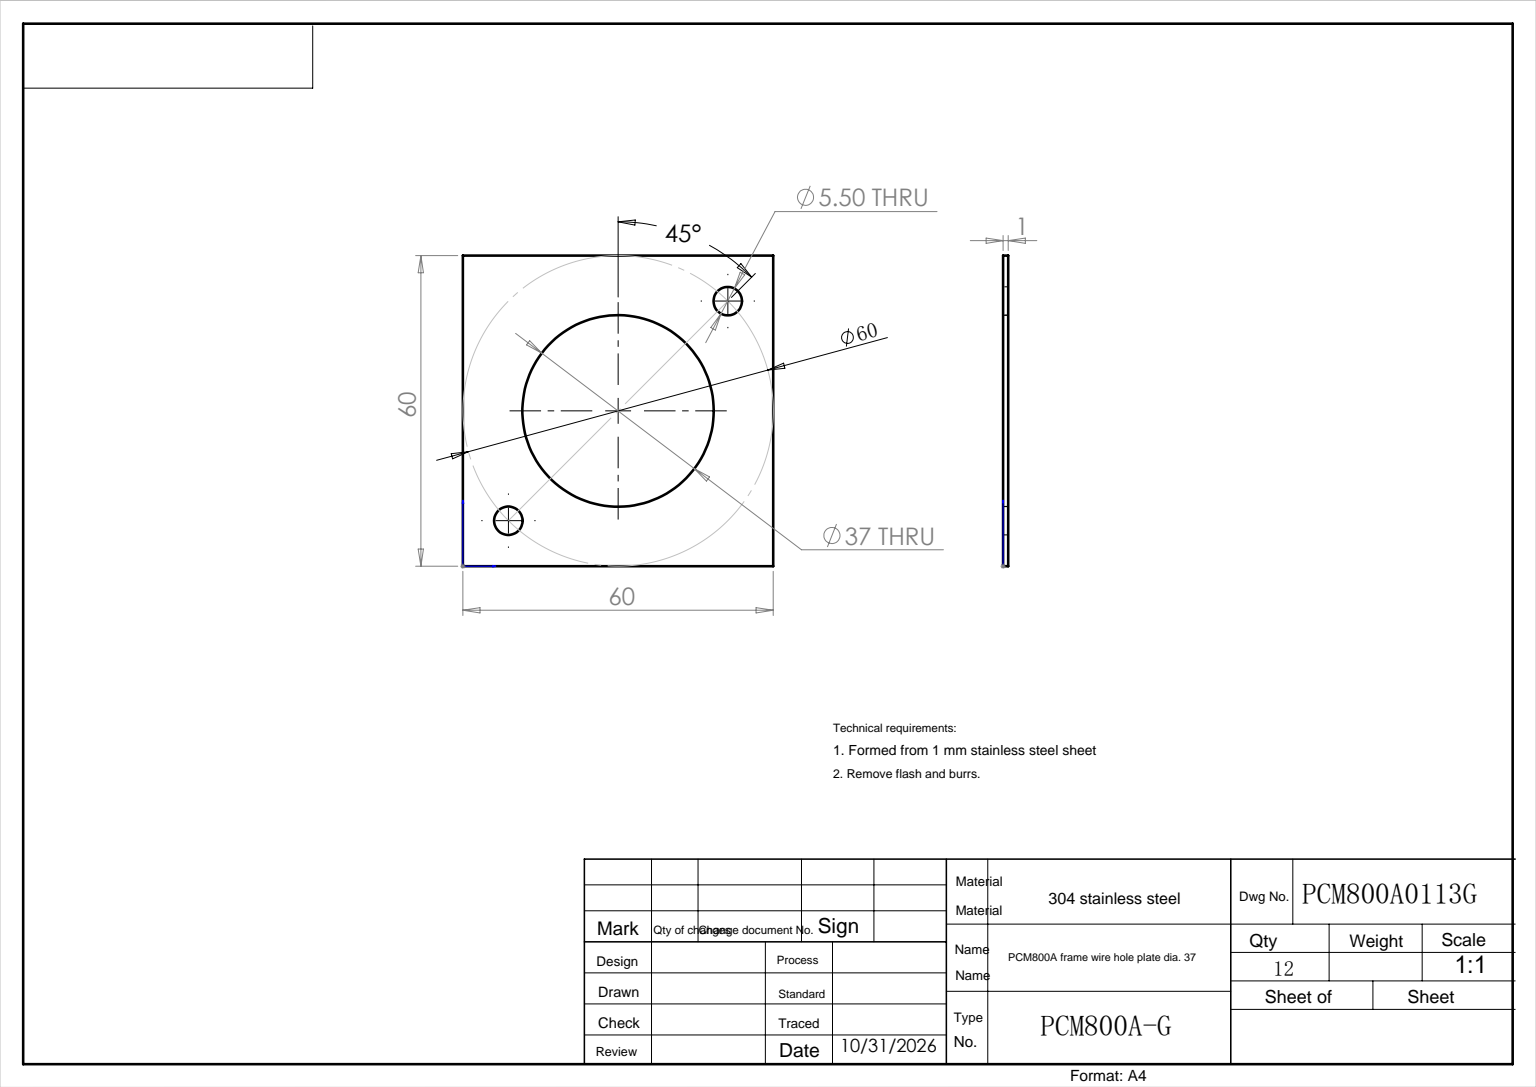
SolidWorks part; units mm, degrees
ref_plane "前视基准面" through (0, 0, 0) normal (0, 0, 1) x (1, 0, 0)
ref_plane "上视基准面" through (0, 0, 0) normal (0, 1, 0) x (1, 0, 0)
ref_plane "右视基准面" through (0, 0, 0) normal (1, 0, 0) x (0, 0, -1)
sketch "草图1" plane through (0, 0, 0) normal (0, 0, 1) x (1, 0, 0)
  line L0 (30, 60) -> (30, -17.1597) construction
  line L1 (0, 0) -> (60, 0)
  line L2 (0, 0) -> (0, 60)
  line L3 (0, 60) -> (60, 60)
  line L4 (60, 0) -> (60, 60)
  line L5 (0, 30) -> (114.8394, 30) construction
  line L6 (0, 0) -> (60, 60) construction
  circle A0 centre (30, 30) radius 18.5
  circle A1 centre (30, 30) radius 30 construction
  circle A2 centre (8.7868, 8.7868) radius 2.75
  circle A3 centre (51.2132, 51.2132) radius 2.75
  dimension "D3" = 37
  dimension "D4" = 60
  dimension "D5" = 5.5
  dimension "D6" = 5.5
  dimension "D1" = 60
  dimension "D2" = 60
extrude "凸台-拉伸1" add sketch "草图1" along normal blind 1
